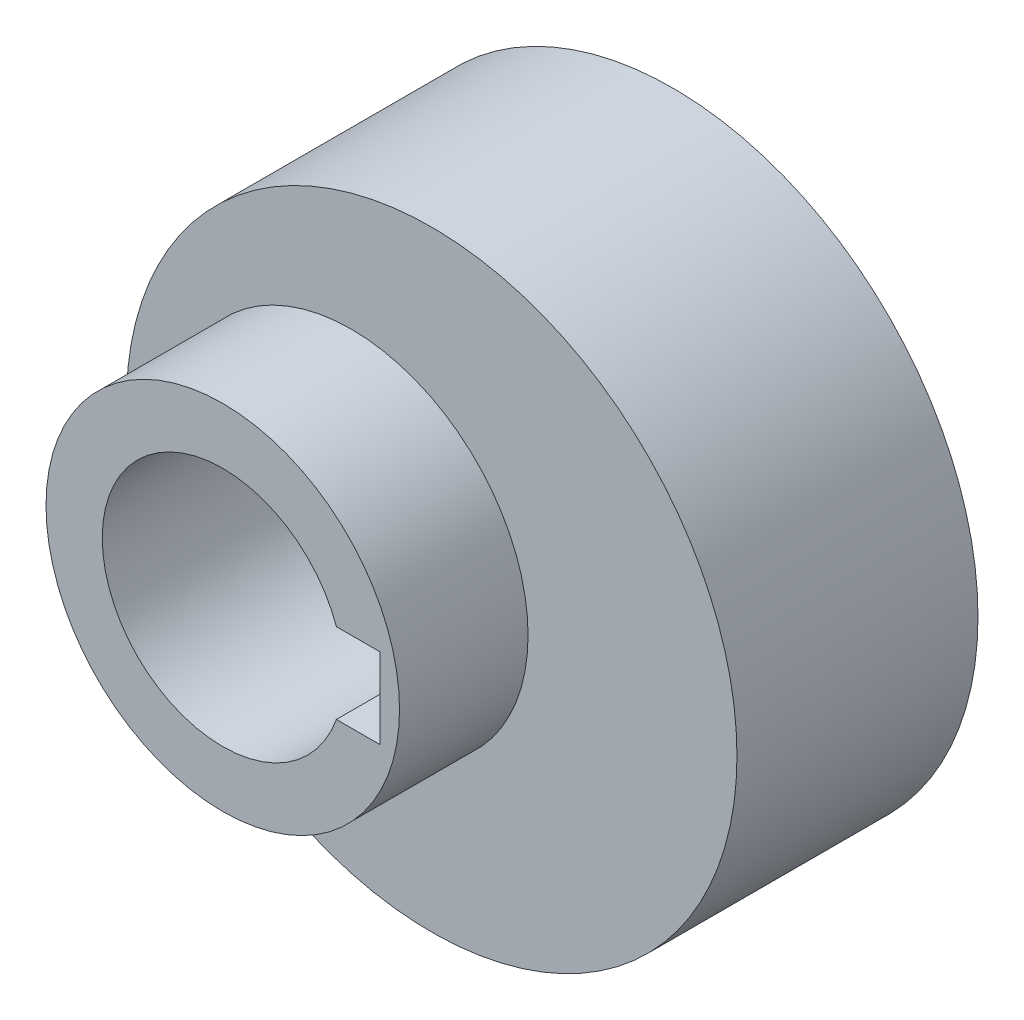
SolidWorks part; units mm, degrees
ref_plane "Front Plane" through (0, 0, 0) normal (0, 0, 1) x (1, 0, 0)
ref_plane "Top Plane" through (0, 0, 0) normal (0, 1, 0) x (1, 0, 0)
ref_plane "Right Plane" through (0, 0, 0) normal (1, 0, 0) x (0, 0, -1)
other "Configuration Table"
sketch "Sketch1" plane through (0, 0, 0) normal (0, 0, 1) x (1, 0, 0)
  circle A0 centre (0, 0) radius 11
  dimension "D1" = 22
extrude "Boss-Extrude1" add sketch "Sketch1" along normal blind 26
sketch "Sketch2" plane through (0, 0, 26) normal (0, 0, 1) x (1, 0, 0)
  line L0 (0, 12.405) -> (0, -12.3425) construction
  line L1 (5, 13.5314) -> (5, -12.0922) construction
  line L2 (-11.9045, 0) -> (15.6588, 0) construction
  circle A0 centre (5, 0) radius 19
  dimension "D3" = 38
  dimension "D1" = 5
  dimension "D2" = 5
extrude "Boss-Extrude2" add sketch "Sketch2" against normal blind 15 from offset 8 offset against normal yes
sketch "Sketch3" plane through (0, 0, 26) normal (0, 0, 1) x (1, 0, 0)
  line L0 (-16.0531, 0) -> (15.6954, 0) construction
  line L1 (7.0711, 2.5) -> (9.8, 2.5)
  line L2 (9.8, 2.5) -> (9.8, -2.5)
  line L3 (9.8, -2.5) -> (7.0711, -2.5)
  arc A0 (7.0711, 2.5) -> (7.0711, -2.5) centre (0, 0) ccw
  dimension "D1" = 15
  dimension "D2" = 5
  dimension "D3" = 2.5
  dimension "D4" = 9.8
extrude "Cut-Extrude1" cut sketch "Sketch3" against normal blind 43
